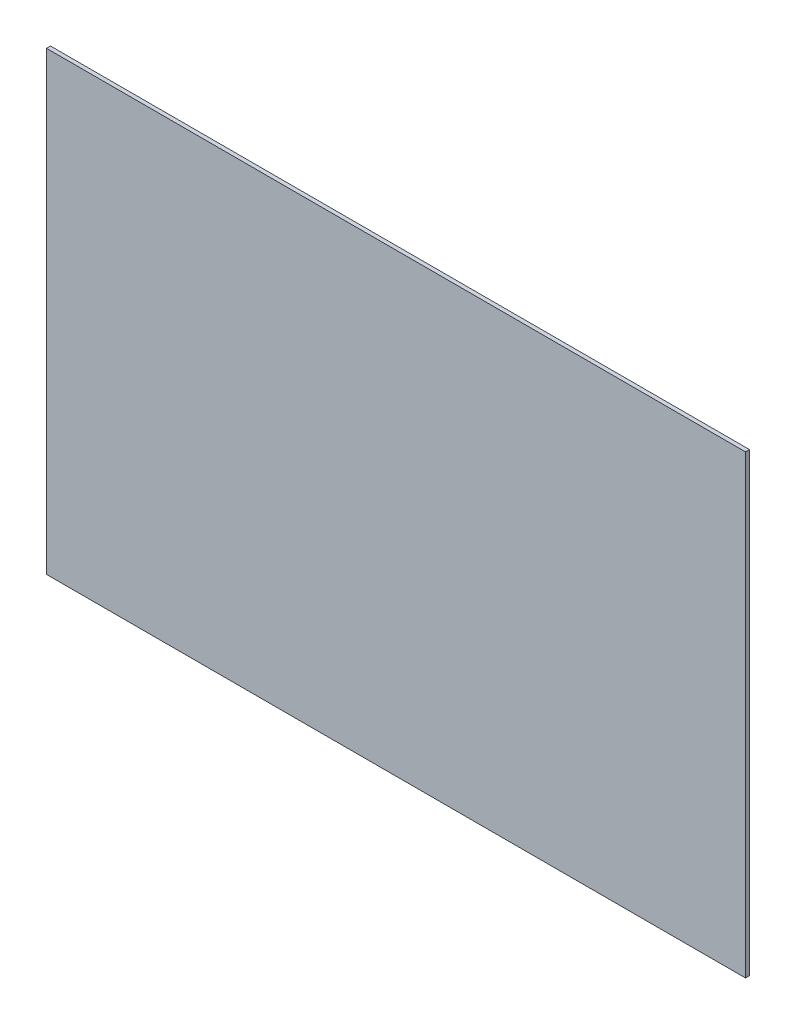
SolidWorks part; units mm, degrees
material "PMMA(有机玻璃)"
ref_plane "前视" through (0, 0, 0) normal (0, 0, 1) x (1, 0, 0)
ref_plane "上视" through (0, 0, 0) normal (0, 1, 0) x (1, 0, 0)
ref_plane "右视" through (0, 0, 0) normal (1, 0, 0) x (0, 0, -1)
sketch "草图1" plane through (0, 0, 0) normal (0, 0, 1) x (1, 0, 0)
  line L1 (-438, 285.5) -> (438, 285.5)
  line L2 (-438, 285.5) -> (-438, -285.5)
  line L3 (-438, -285.5) -> (438, -285.5)
  line L4 (438, 285.5) -> (438, -285.5)
  line L5 (-438, 285.5) -> (438, -285.5) construction
  line L6 (-438, -285.5) -> (438, 285.5) construction
  point P0 (0, 0)
  dimension "D1" = 571
  dimension "D2" = 876
extrude "凸台-拉伸1" add sketch "草图1" along normal blind 5
hole_wizard "M5 间隙孔1" positions "草图3" profile "草图2" hole size "M5" standard "GB"
sketch "草图3" plane through (0, 0, 5) normal (0, 0, 1) x (1, 0, 0)
  line L0 (-427.5, 273) -> (-427.5, -273) construction
  line L1 (-427.5, -273) -> (427.5, -273) construction
  line L2 (0, 273) -> (0, -273) construction
  line L3 (427.5, 273) -> (-427.5, 273) construction
  line L5 (-427.5, 0) -> (427.5, 0) construction
  line L6 (427.5, -273) -> (427.5, 273) construction
  point P0 (-375, -261)
  point P46 (415.5, 250)
  point P48 (-415.5, 250)
  point P58 (-125, -261)
  point P59 (125, -261)
  point P61 (-125, 261)
  point P62 (125, 261)
  point P64 (-375, 261)
  point P88 (375, -261)
  point P89 (375, 261)
  point P108 (415.5, 0)
  point P109 (-415.5, 0)
  point P110 (415.5, -250)
  point P111 (-415.5, -250)
  dimension "D1" = 12
  dimension "D2" = 12
  dimension "D5" = 3
  dimension "D3" = 12
  dimension "D6" = 4
  dimension "D4" = 2
sketch "草图2" plane through (-375, -261, 5) normal (1, 0, 0) x (0, -1, 0)
  line L0 (0, 0) -> (0, 5)
  line L1 (0, 5) -> (2.75, 5)
  line L2 (2.75, 5) -> (2.75, 0)
  line L5 (2.75, 0) -> (0, 0)
  line L11 (0, -6.35) -> (0, 107.95) construction
  dimension "通孔孔直径" = 5.5
  dimension "通孔孔深度" = 5
